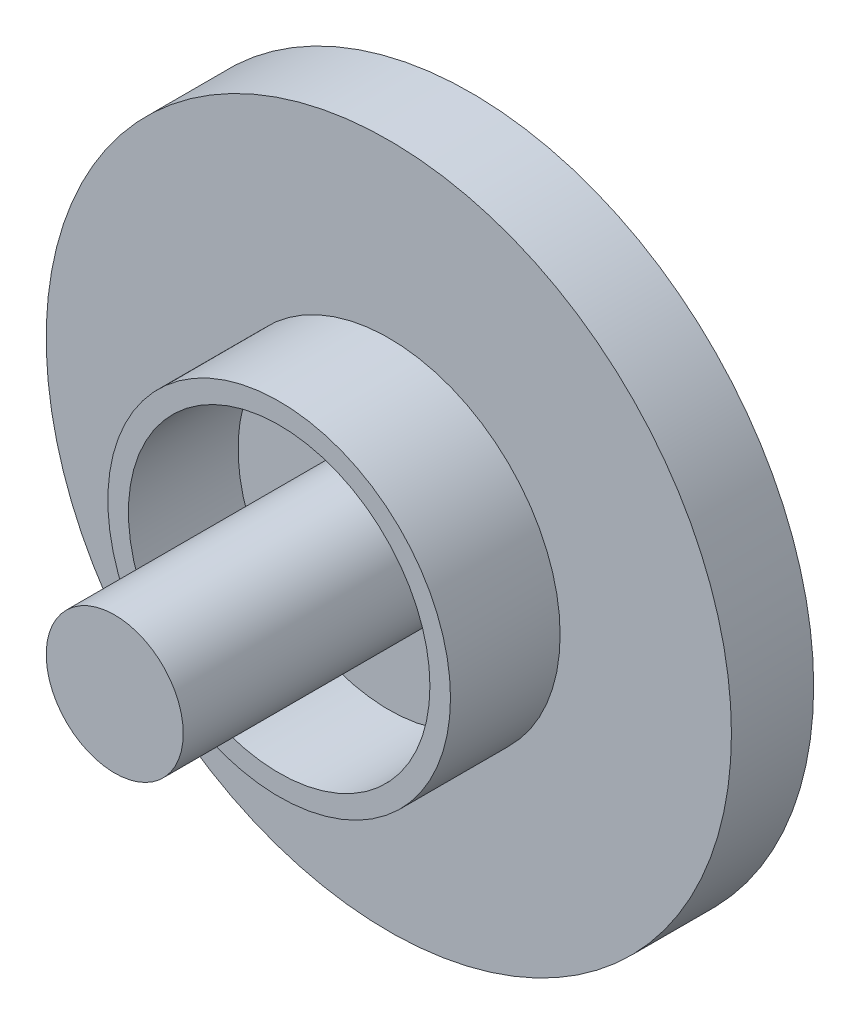
from build123d import *

# Parameters (mm, degrees)
SKETCH_1_R      = 25
EXTRUDE_1_DEPTH = 6
SKETCH_2_R      = 12.5
SKETCH_2_R_2    = 11
EXTRUDE_2_DEPTH = 8
SKETCH_3_R      = 5
EXTRUDE_3_DEPTH = 20
SKETCH_5_R      = 11.5
SKETCH_5_R_2    = 10.475
EXTRUDE_4_DEPTH = 4
SKETCH_6_R      = 1.425
EXTRUDE_5_DEPTH = 10


with BuildPart() as part:
    # 草图1 → 凸台-拉伸1 (new body)
    with BuildSketch(Plane.XY):
        Circle(SKETCH_1_R)
    extrude(amount=EXTRUDE_1_DEPTH)

    # 草图2 → 凸台-拉伸2 (add)
    with BuildSketch(Plane.XY.offset(6)):
        Circle(SKETCH_2_R)
        Circle(SKETCH_2_R_2, mode=Mode.SUBTRACT)
    extrude(amount=EXTRUDE_2_DEPTH)

    # 草图3 → 凸台-拉伸3 (add)
    with BuildSketch(Plane.XY.offset(6)):
        Circle(SKETCH_3_R)
    extrude(amount=EXTRUDE_3_DEPTH)

    # 草图5 → 凸台-拉伸4 (add)
    with BuildSketch(Plane(origin=(0, 0, 0), x_dir=(-1, 0, 0), z_dir=(0, 0, -1))):
        with Locations(Location((0, 0, 0), (0, 0, 180))):
            Circle(SKETCH_5_R)
        Circle(SKETCH_5_R_2, mode=Mode.SUBTRACT)
    extrude(amount=EXTRUDE_4_DEPTH)

    # 草图6 → 凸台-拉伸5 (add)
    with BuildSketch(Plane(origin=(0, 0, 0), x_dir=(-1, 0, 0), z_dir=(0, 0, -1))):
        with Locations(Location((0, 0, 0), (0, 0, 180))):
            Circle(SKETCH_6_R)
    extrude(amount=EXTRUDE_5_DEPTH)


solid = part.part
